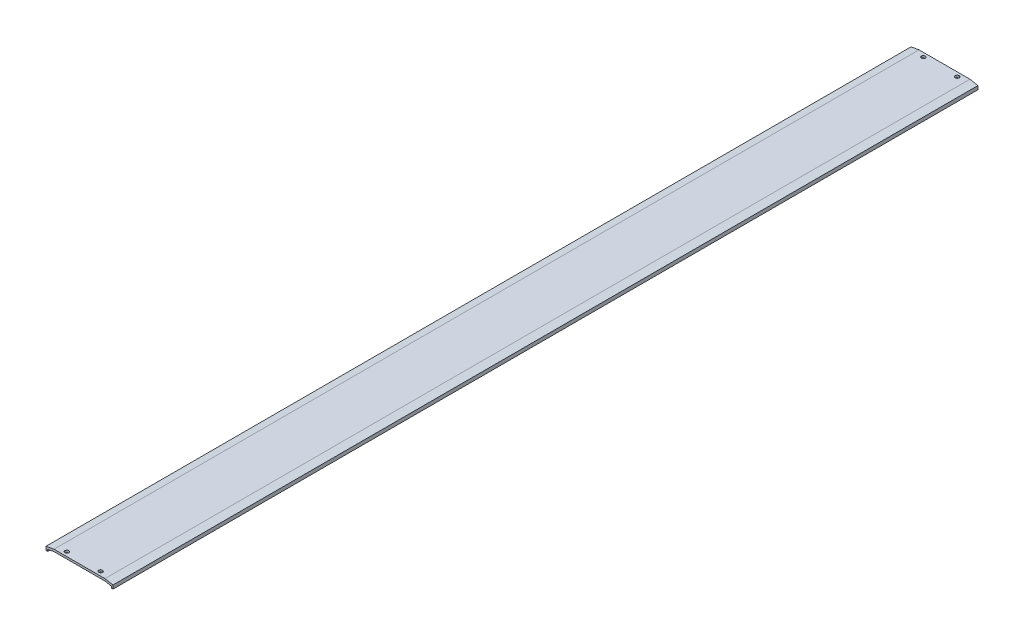
SolidWorks part; units mm, degrees
material "6061 合金"
ref_plane "前视基准面" through (0, 0, 0) normal (0, 0, 1) x (1, 0, 0)
ref_plane "上视基准面" through (0, 0, 0) normal (0, 1, 0) x (1, 0, 0)
ref_plane "右视基准面" through (0, 0, 0) normal (1, 0, 0) x (0, 0, -1)
sketch "草图1" plane through (0, 0, 0) normal (0, 0, 1) x (1, 0, 0)
  line L0 (0, 0) -> (0, 49.2018) construction
  line L1 (-37.5, 0) -> (-39.5, 0)
  line L2 (-39.5, 0) -> (-39.5, 4.3)
  line L3 (-39.5, 4.3) -> (-30, 6)
  line L4 (-30, 6) -> (30, 6)
  line L5 (-37.5, 0) -> (-37.5, 2.1221)
  line L6 (-37.5, 2.1221) -> (-29.8, 3.5)
  line L7 (-29.8, 3.5) -> (29.8, 3.5)
  line L8 (37.5, 2.1221) -> (29.8, 3.5)
  line L9 (37.5, 0) -> (37.5, 2.1221)
  line L10 (39.5, 4.3) -> (30, 6)
  line L11 (39.5, 0) -> (39.5, 4.3)
  line L12 (37.5, 0) -> (39.5, 0)
  point P12 (0, 3.5)
  point P15 (0, 6)
  dimension "D1" = 79
  dimension "D2" = 75
  dimension "D3" = 2.5
  dimension "D4" = 4.3
  dimension "D5" = 6
  dimension "D6" = 59.6
  dimension "D7" = 60
extrude "凸台-拉伸1" add sketch "草图1" along normal mid plane 1020
sketch "草图2" plane through (0, 6, 0) normal (0, 1, 0) x (1, 0, 0)
  line L0 (30, 510) -> (-30, 510) construction
  line L1 (0, 0) -> (0, 625.3792) construction
  circle A0 centre (-20, 505) radius 2.25
  circle A1 centre (20, 505) radius 2.25
  dimension "D1" = 4.5
  dimension "D2" = 5
  dimension "D3" = 40
extrude "切除-拉伸1" cut sketch "草图2" against normal blind 20
mirror "镜向1" about plane through (0, 0, 0) normal (0, 0, 1) of "切除-拉伸1"
